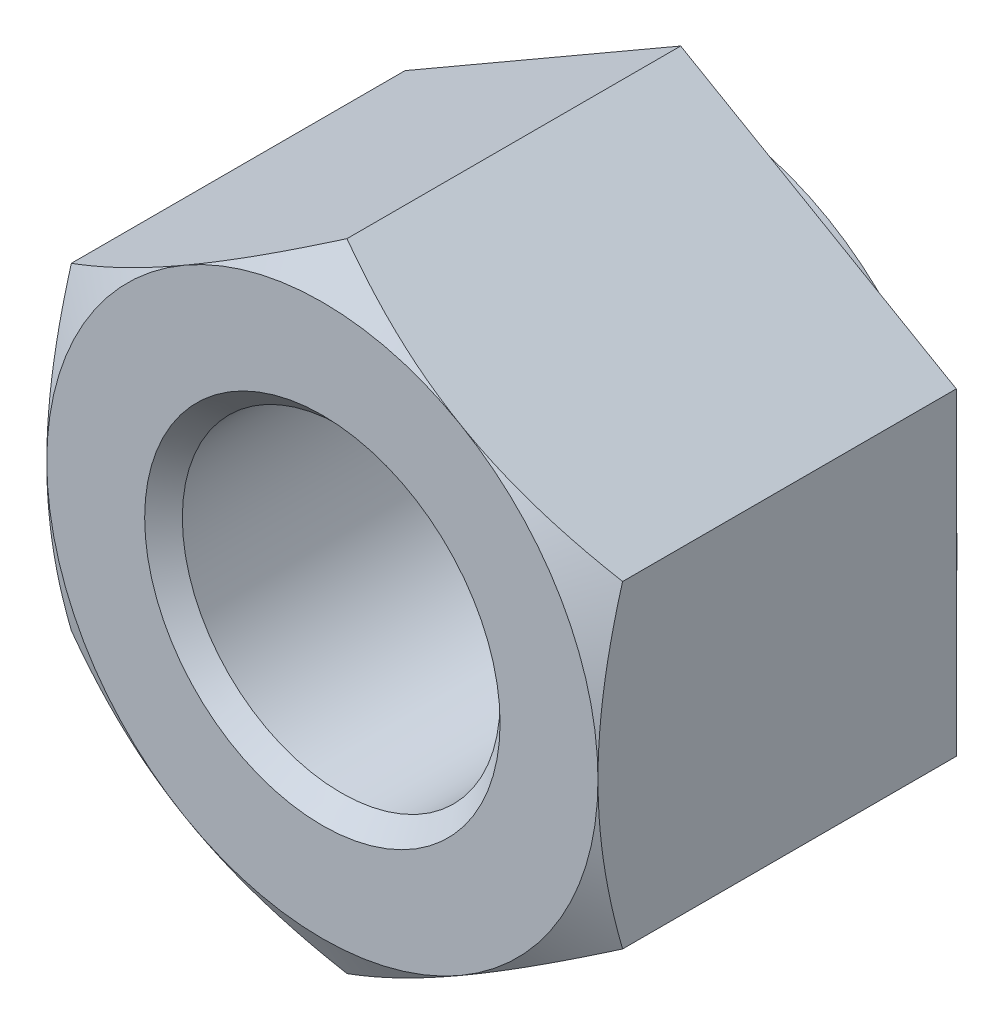
SolidWorks part; units mm, degrees
ref_plane "Front Plane" through (0, 0, 0) normal (0, 0, 1) x (1, 0, 0)
ref_plane "Top Plane" through (0, 0, 0) normal (0, 1, 0) x (1, 0, 0)
ref_plane "Right Plane" through (0, 0, 0) normal (1, 0, 0) x (0, 0, -1)
sketch "Dimension Sketch" plane through (0, 0, 0) normal (0, 0, 1) x (1, 0, 0)
  line L0 (0, 0) -> (16, 0) construction
  point P3 (17.3, 0)
  point P4 (2, 0)
  point P5 (0.8, 0)
  point P6 (22.5, 0)
  point P7 (26.75, 0)
  point P8 (16.4, 0)
  point P9 (12.6, 0)
  point P10 (24, 0)
  dimension "D" = 16
  dimension "da(最大)" = 17.3
  dimension "P" = 2
  dimension "c(最大)" = 0.8
  dimension "dw(最小)" = 22.5
  dimension "e(最小)" = 26.75
  dimension "m(最大)" = 16.4
  dimension "m´(最小)" = 12.6
  dimension "s(最大)" = 24
sketch "Sketch1" plane through (0, 0, 0) normal (0, 0, 1) x (1, 0, 0)
  line L1 (0, 13.8564) -> (-12, 6.9282)
  line L2 (-12, 6.9282) -> (-12, -6.9282)
  line L3 (-12, -6.9282) -> (0, -13.8564)
  line L4 (0, -13.8564) -> (12, -6.9282)
  line L5 (12, -6.9282) -> (12, 6.9282)
  line L6 (12, 6.9282) -> (0, 13.8564)
  circle A0 centre (0, 0) radius 12 construction
  circle A1 centre (0, 0) radius 6.9175
  dimension "dm" = 13.835
  dimension "s" = 24
extrude "Extrude1" add sketch "Sketch1" along normal blind 16.4
cosmetic thread "Cosmetic Thread1" parameters "D2"=16
sketch "Sketch2" plane through (0, 0, 0) normal (0, 0, 1) x (1, 0, 0)
  circle A0 centre (0, 0) radius 11.25
  dimension "dw" = 22.5
extrude "Cut-Extrude2" cut sketch "Sketch2" along normal blind 0.8 flip side to cut
sketch "Sketch3" plane through (0, 0, 16.4) normal (0, 0, 1) x (1, 0, 0)
  line L0 (0, -13.8564) -> (12, -6.9282) construction
  circle A0 centre (0, 0) radius 12
extrude "Cut-Extrude3" cut sketch "Sketch3" against normal through all draft 60 flip side to cut
chamfer "Chamfer1" distance 0.82 angle 45 2 edges at (6.9175, 0, 0) (6.9175, 0, 16.4)
